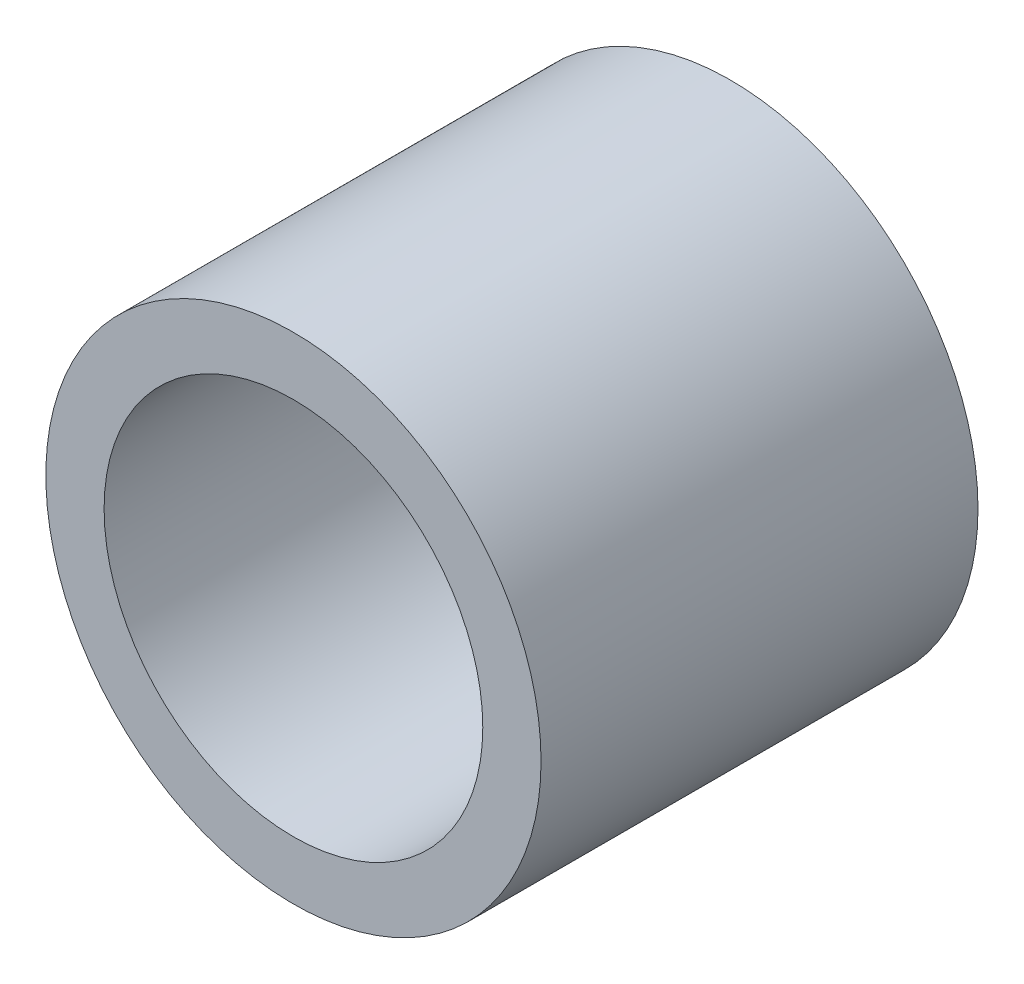
SolidWorks part; units mm, degrees
material "Q235-A"
ref_plane "前视基准面" through (0, 0, 0) normal (0, 0, 1) x (1, 0, 0)
ref_plane "上视基准面" through (0, 0, 0) normal (0, 1, 0) x (1, 0, 0)
ref_plane "右视基准面" through (0, 0, 0) normal (1, 0, 0) x (0, 0, -1)
sketch "草图1" plane through (0, 0, 0) normal (0, 0, 1) x (1, 0, 0)
  circle A0 centre (0, 0) radius 34
  circle A1 centre (0, 0) radius 26
  dimension "D1" = 52
  dimension "D2" = 68
extrude "凸台-拉伸1" add sketch "草图1" along normal blind 60
